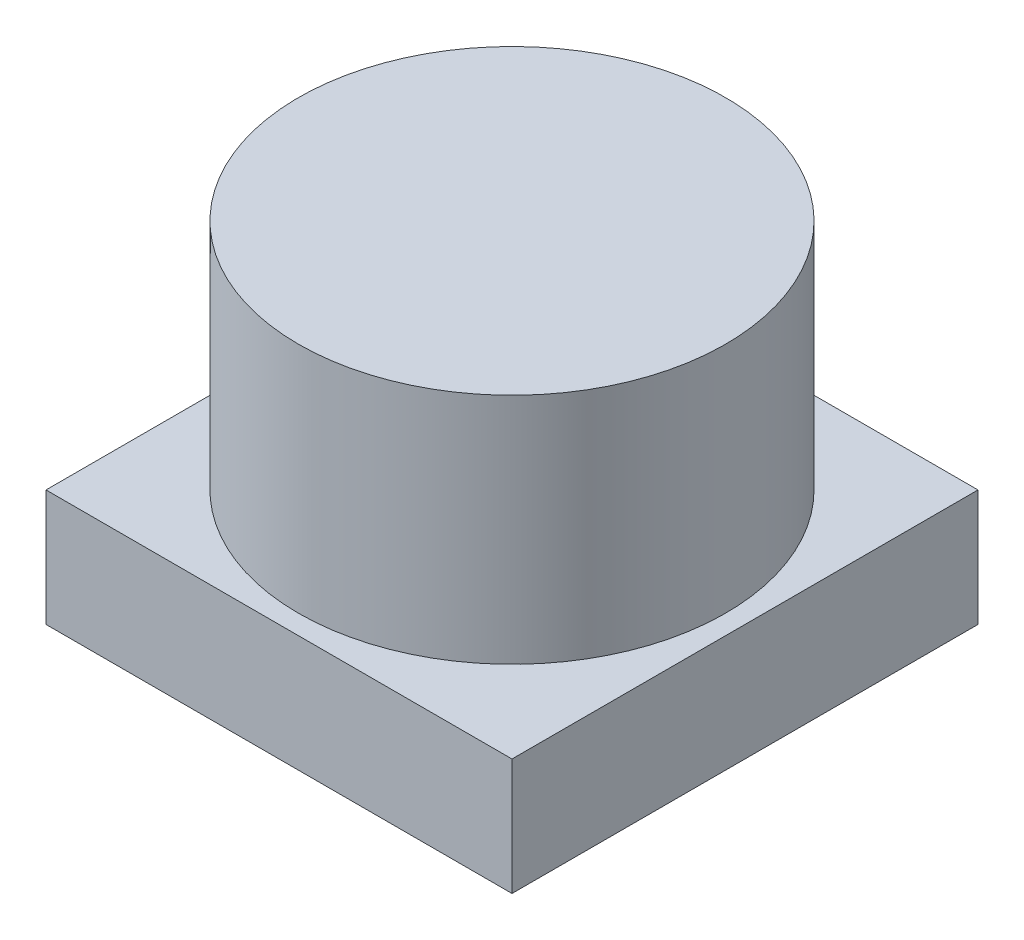
SolidWorks part; units mm, degrees
ref_plane "Front Plane" through (0, 0, 0) normal (0, 0, 1) x (1, 0, 0)
ref_plane "Top Plane" through (0, 0, 0) normal (0, 1, 0) x (1, 0, 0)
ref_plane "Right Plane" through (0, 0, 0) normal (1, 0, 0) x (0, 0, -1)
sketch "Sketch1" plane through (0, 0, 0) normal (0, 1, 0) x (1, 0, 0)
  circle A0 centre (0, 0) radius 2.75
  dimension "D1" = 5.5
extrude "Boss-Extrude1" add sketch "Sketch1" along normal blind 3
sketch "Sketch2" plane through (0, 0, 0) normal (0, -1, 0) x (1, 0, 0)
  line L1 (-3, -3) -> (3, -3)
  line L2 (-3, -3) -> (-3, 3)
  line L3 (-3, 3) -> (3, 3)
  line L4 (3, -3) -> (3, 3)
  line L5 (-3, -3) -> (3, 3) construction
  line L6 (-3, 3) -> (3, -3) construction
  point P0 (0, 0)
  dimension "D1" = 6
  dimension "D2" = 6
extrude "Boss-Extrude2" add sketch "Sketch2" along normal blind 1.5
